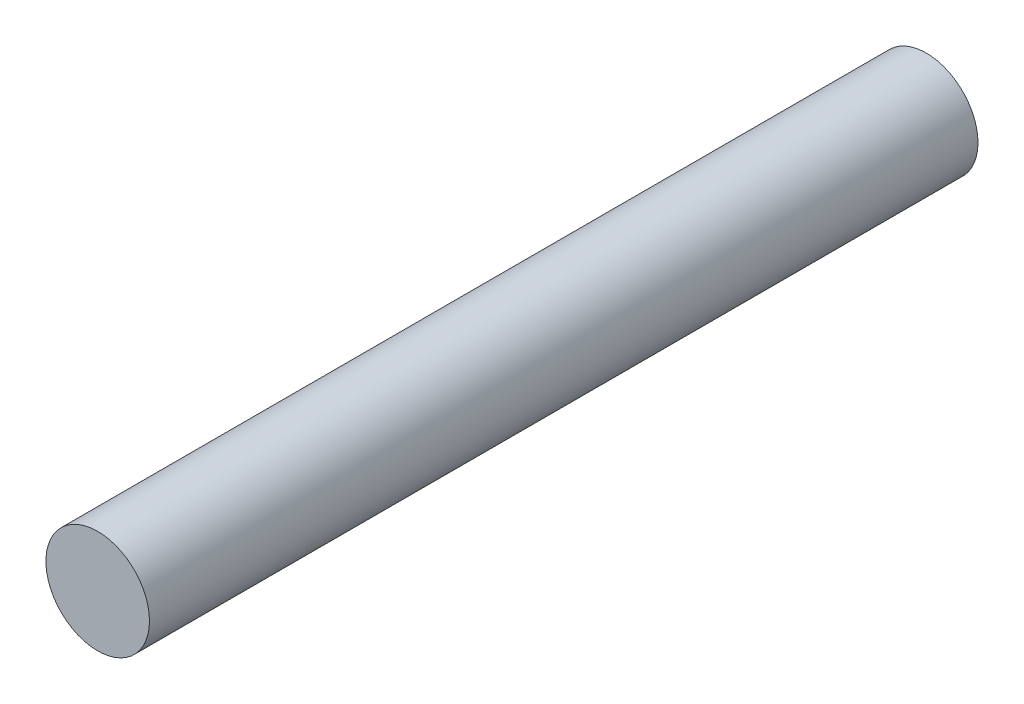
SolidWorks part; units mm, degrees
ref_plane "Front Plane" through (0, 0, 0) normal (0, 0, 1) x (1, 0, 0)
ref_plane "Top Plane" through (0, 0, 0) normal (0, 1, 0) x (1, 0, 0)
ref_plane "Right Plane" through (0, 0, 0) normal (1, 0, 0) x (0, 0, -1)
other "Configuration Table"
sketch "Sketch2" plane through (0, 0, 0) normal (0, 0, 1) x (1, 0, 0)
  circle A0 centre (0, 0) radius 15
extrude "Boss-Extrude1" add sketch "Sketch2" against normal blind 40 and the other way blind 200
